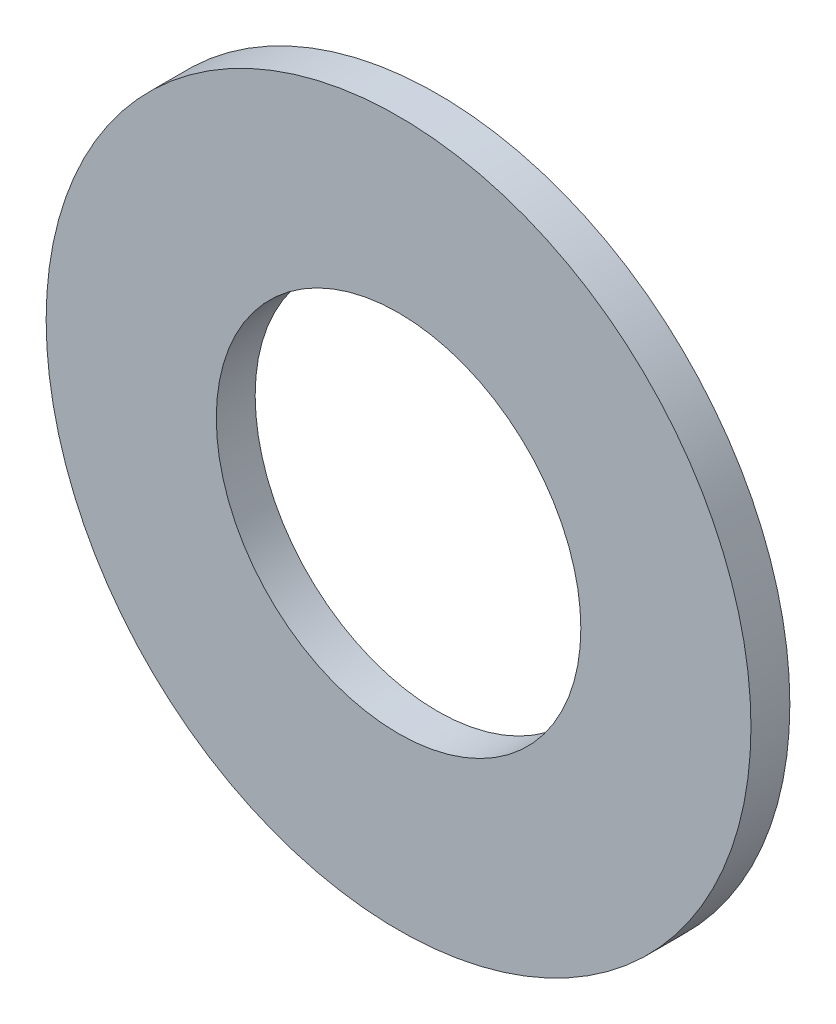
SolidWorks part; units mm, degrees
ref_plane "前视基准面" through (0, 0, 0) normal (0, 0, 1) x (1, 0, 0)
ref_plane "上视基准面" through (0, 0, 0) normal (0, 1, 0) x (1, 0, 0)
ref_plane "右视基准面" through (0, 0, 0) normal (1, 0, 0) x (0, 0, -1)
sketch "草图1" plane through (0, 0, 0) normal (0, 0, 1) x (1, 0, 0)
  circle A0 centre (0, 0) radius 15
  circle A1 centre (0, 0) radius 29
  dimension "D1" = 30
  dimension "D2" = 58
extrude "凸台-拉伸1" add sketch "草图1" along normal blind 3.2
